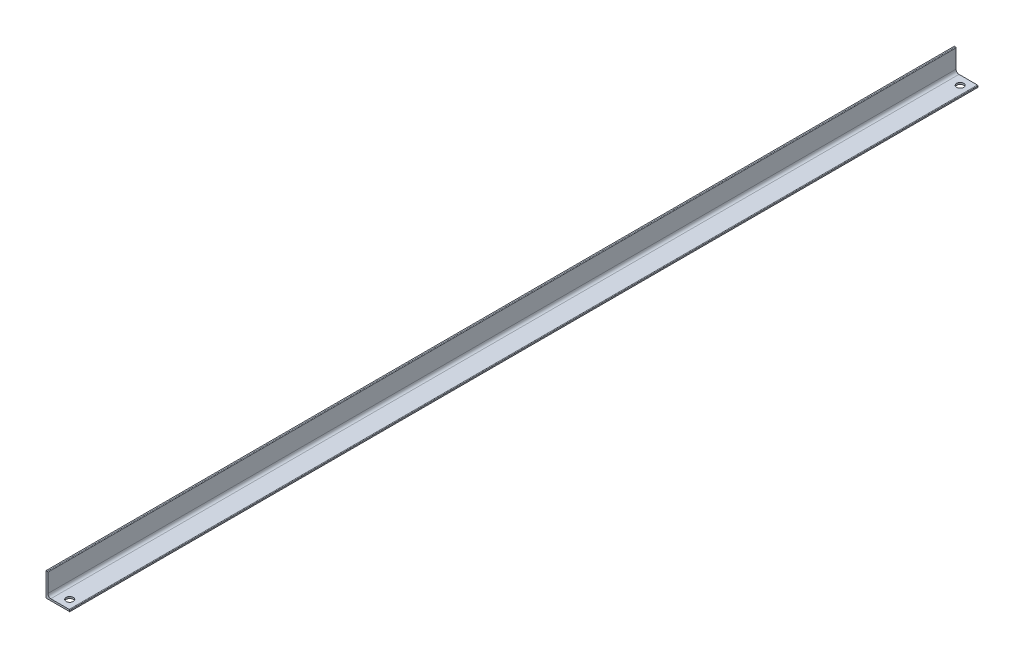
SolidWorks part; units mm, degrees
material "Q235B"
ref_plane "Plane1" through (0, 0, 0) normal (0, 0, 1) x (1, 0, 0)
ref_plane "Plane2" through (0, 0, 0) normal (0, 1, 0) x (1, 0, 0)
ref_plane "Plane3" through (0, 0, 0) normal (1, 0, 0) x (0, 0, -1)
sketch "Sketch1" plane through (0, 0, 0) normal (0, 0, 1) x (1, 0, 0)
  line L0 (0, 0) -> (0, 40)
  line L1 (0, 20) -> (3, 20) construction
  line L2 (3, 39) -> (3, 8)
  line L3 (8, 3) -> (39, 3)
  line L4 (20, 3) -> (20, 0) construction
  line L5 (40, 0) -> (0, 0)
  line L6 (0, 40) -> (2, 40)
  line L7 (40, 0) -> (40, 2)
  arc A0 (40, 2) -> (39, 3) centre (39, 2) ccw
  arc A1 (2, 40) -> (3, 39) centre (2, 39) cw
  arc A2 (8, 3) -> (3, 8) centre (8, 8) cw
  point P10 (20, 0)
  point P14 (0, 20)
  point P15 (3, 20)
  point P16 (20, 3)
  point P17 (3, 40)
  point P18 (40, 3)
  point P21 (40, 3)
  point P24 (3, 40)
extrude "Boss-Extrude1" add sketch "Sketch1" along normal blind 1530 contours L5 L0 L6 A1 L2 A2 L3 A0 L7
sketch "草图1" plane through (0, 0, 0) normal (0, -1, 0) x (1, 0, 0)
  line L0 (40, 1530) -> (0, 1530) construction
  line L1 (40, 1530) -> (40, 0) construction
  line L2 (40, 0) -> (0, 0) construction
  circle A0 centre (25, 1515) radius 6
  circle A1 centre (25, 15) radius 6
  dimension "D1" = 12
  dimension "D2" = 15
  dimension "D3" = 15
  dimension "D4" = 15
  dimension "D5" = 15
extrude "Cut-Extrude1" cut sketch "草图1" against normal through all
equation "\"D2@Sketch1\" = \"D1@Sketch1\" / 3"
